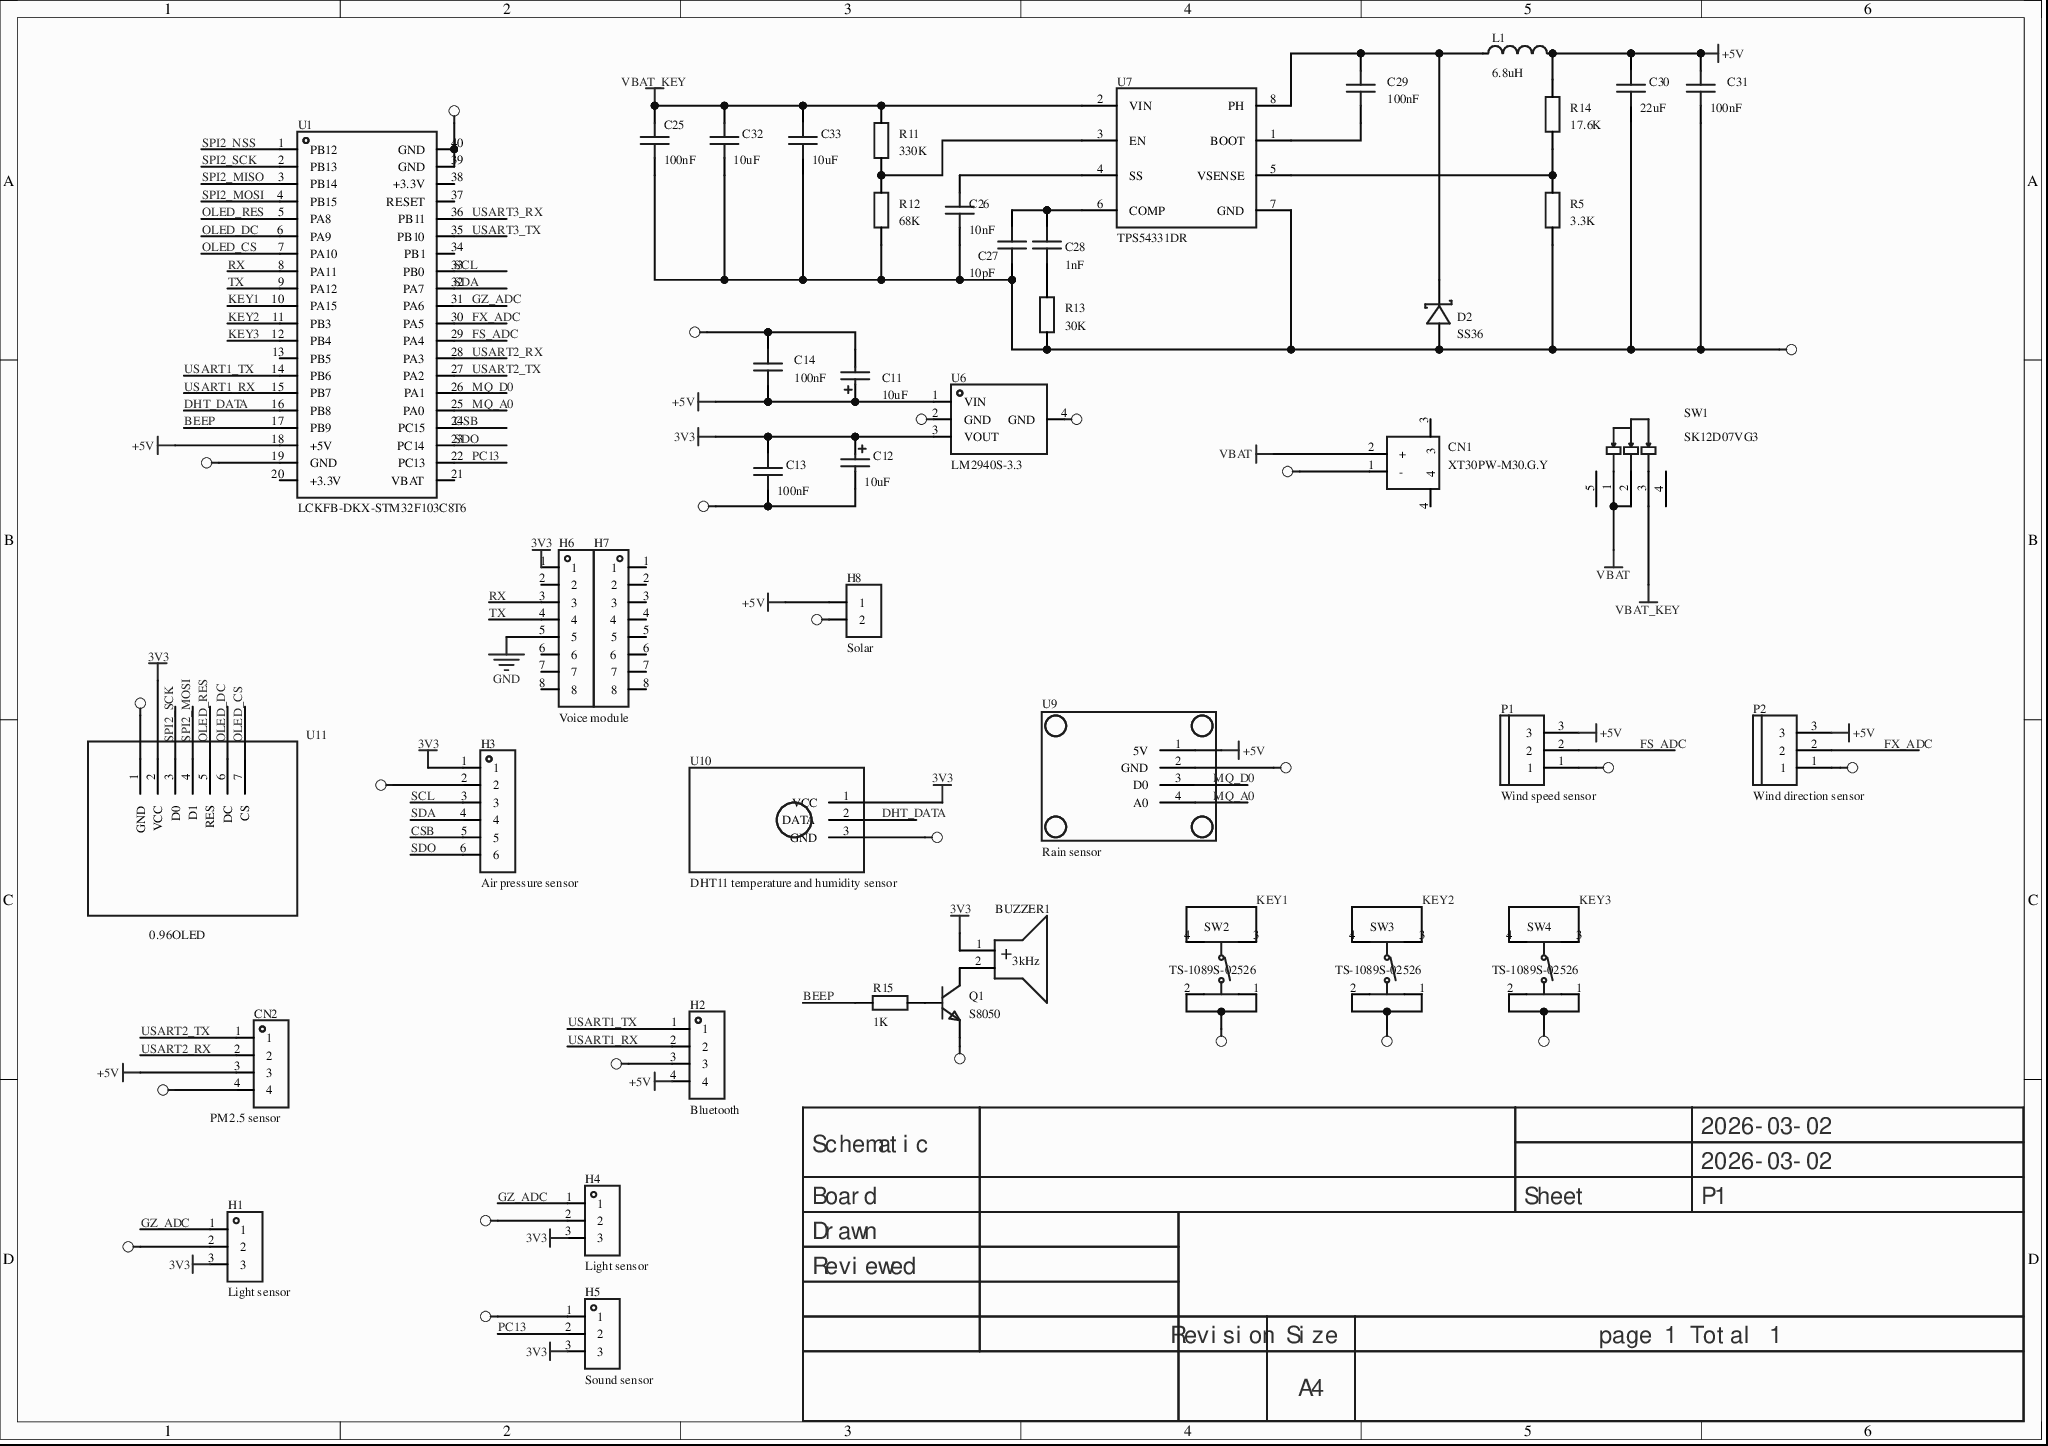
[diagram p0: MISC64781-3.schdoc]
# Altium project MISC64781-2.PrjPcb
1 sheet, 45 parts. Net scope: global (net labels, ports and power ports of the same name join across sheets).
Board file: MISC64781.pcbdoc

## Sheet MISC64781-3.schdoc
size 297 x 209 mm; Version: V1.0; @Project Name: MISC64781; @Page Count: 1; @Update Date: 2026-03-02; @Create Date: 2026-03-02; @Schematic Name: MISC64781; @Page No: 1; @Create Time: 18:43:32; @Update Time: 20:38:21; @Board Name: MISC64781

### Parts
BUZZER1  3kHz  [BUZ-TH_BD9.0-P5.00-D0.6-FD]
C11  10uF  [CASE-A_3216]
C12  10uF  [CASE-A_3216]
C13  100nF  [C0603]
C14  100nF  [C0603]
C25  100nF  [C0603]
C26  10nF  [C0603]
C27  10pF  [C0603]
C28  1nF  [C0603]
C29  100nF  [C0603]
C30  22uF  [C0603]
C31  100nF  [C0603]
C32  10uF  [C0805]
C33  10uF  [C0805]
CN1  XT30PW-M30.G.Y  [CONN-TH_XT30PW-M]
CN2  PM2.5 sensor  [CONN-TH_4P-P1.50_HCTL_HC-ZH1.5-4AW]
D2  SS36  [SMA_L4.3-W2.6-LS5.2-RD]
H1  Light sensor  [HDR-TH_3P-P2.54-V-F]
H2  Bluetooth  [HDR-TH_4P-P2.54-V-F]
H3  Air pressure sensor  [HDR-TH_6P-P2.54-V-F]
H4  Light sensor  [HDR-TH_3P-P2.54-V-F]
H5  Sound sensor  [HDR-TH_3P-P2.54-V-F]
H6  Voice module  [HDR-TH_8P-P2.54-V-F-1]
H7  (no value)  [HDR-TH_8P-P2.54-V-F-1]
H8  Solar  [HDR-TH_2P-P2.54-V-F]
L1  6.8uH  [IND-SMD_L7.0-W6.6]
P1  Wind speed sensor  [CONN-TH_3P-P5.00_WJ500V-5.08-3P]
P2  Wind direction sensor  [CONN-TH_3P-P5.00_WJ500V-5.08-3P]
Q1  S8050  [SOT-23-3_L2.9-W1.3-P1.90-LS2.3-BR]
R5  3.3K  [R0603]
R11  330K  [R0603]
R12  68K  [R0603]
R13  30K  [R0603]
R14  17.6K  [R0603]
R15  1K  [R0603]
SW1  SK12D07VG3  [SW-TH_SK12D07VG3]
SW2  TS-1089S-02526  [SW-SMD_4P-L4.2-W3.3-P2.15-LS5.1]
SW3  TS-1089S-02526  [SW-SMD_4P-L4.2-W3.3-P2.15-LS5.1]
SW4  TS-1089S-02526  [SW-SMD_4P-L4.2-W3.3-P2.15-LS5.1]
U1  LCKFB-DKX-STM32F103C8T6  [CONN-TH_L53.3-W22.9_STM32F103C8T6-CARD]
U6  LM2940S-3.3  [SOT-223-3_L6.5-W3.4-P2.30-LS7.0-BR]
U7  TPS54331DR  [SOIC-8_L5.0-W4.0-P1.27-LS6.0-BL]
U9  Rain sensor  [MQ-2烟雾传感器模块]
U10  DHT11 temperature and humidity sensor  [DHT11温湿度模块]
U11  0.96OLED  [0.96寸OLED]

### Nets
3V3: BUZZER1.1(+) C12.1 C13.2 H1.3 H3.1 H4.3 H5.3 H6.1 U6.3(VOUT) U10.1(VCC) U11.2(VCC)
+5V: C11.1 C14.1 C30.2 C31.2 CN2.3 H2.4 H8.1 L1.2 P1.3 P2.3 R14.2 U1.18(+5V) U6.1(VIN) U9.1(5V)
GND: H6.5
PGND: C11.2 C12.2 C13.1 C14.2 C25.1 C26.1 C27.1 C30.1 C31.1 C32.1 C33.1 CN1.1(-) CN2.4 D2.2(A) H1.2 H2.3 H3.2 H4.2 H5.1 H8.2 P1.1 P2.1 Q1.2(E) R5.1 R12.1 R13.1 SW2.1 SW2.2 SW3.1 SW3.2 SW4.1 SW4.2 U1.19(GND) U1.39(GND) U1.40(GND) U6.2(GND) U6.4(GND) U7.7(GND) U9.2(GND) U10.3(GND) U11.1(GND)
VBAT: CN1.2(+) SW1.1 SW1.2
VBAT_KEY: C25.2 C32.2 C33.2 R11.2 SW1.3 U7.2(VIN)
BEEP: R15.1 U1.17(PB9)
CSB: H3.5 U1.24(PC15)
DHT_DATA: U1.16(PB8) U10.2(DATA)
FS_ADC: P1.2 U1.29(PA4)
FX_ADC: P2.2 U1.30(PA5)
GZ_ADC: H1.1 H4.1 U1.31(PA6)
KEY1: SW2.3 SW2.4 U1.10(PA15)
KEY2: SW3.3 SW3.4 U1.11(PB3)
KEY3: SW4.3 SW4.4 U1.12(PB4)
MQ_A0: U1.25(PA0) U9.4(A0)
MQ_D0: U1.26(PA1) U9.3(D0)
OLED_CS: U1.7(PA10) U11.7(CS)
OLED_DC: U1.6(PA9) U11.6(DC)
OLED_RES: U1.5(PA8) U11.5(RES)
PC13: H5.2 U1.22(PC13)
RX: H6.3 U1.8(PA11)
SCL: H3.3 U1.33(PB0)
SDA: H3.4 U1.32(PA7)
SDO: H3.6 U1.23(PC14)
SPI2_MISO: U1.3(PB14)
SPI2_MOSI: U1.4(PB15) U11.4(D1)
SPI2_NSS: U1.1(PB12)
SPI2_SCK: U1.2(PB13) U11.3(D0)
TX: H6.4 U1.9(PA12)
USART1_RX: H2.2 U1.15(PB7)
USART1_TX: H2.1 U1.14(PB6)
USART2_RX: CN2.2 U1.28(PA3)
USART2_TX: CN2.1 U1.27(PA2)
USART3_RX: U1.36(PB11)
USART3_TX: U1.35(PB10)
NetBUZZER1_2: BUZZER1.2(-) Q1.3(C)
NetC26_2: C26.2 U7.4(SS)
NetC27_2: C27.2 C28.2 U7.6(COMP)
NetC28_1: C28.1 R13.2
NetC29_1: C29.1 U7.1(BOOT)
NetC29_2: C29.2 D2.1(K) L1.1 U7.8(PH)
NetQ1_1: Q1.1(B) R15.2
NetR5_2: R5.2 R14.1 U7.5(VSENSE)
NetR11_1: R11.1 R12.2 U7.3(EN)

Not connected (* = marked no-connect by the designer): CN1 3* 4*; H6 2 6 7 8; H7 1 2 3 4 5 6 7 8; SW1 4* 5*; U1 13(PB5) 20(+3.3V)* 21(VBAT)* 34(PB1) 37(RESET)* 38(+3.3V)*

### Notes on the sheet
- 2026-03-02
- Schematic
- Board
- Sheet
- P1
- Drawn
- Reviewed
- Revision
- Size
- A4
- page 1 Total 1

### Library data of the parts
BUZZER1 = HNB09A03: Drive: active (built-in driver circuit); type: electromagnetic; frequency: 3kHz; SPL: 85dB;; Manufacturer: 华能; AddInBom: yes; ModelId: 13273335caac486e928bafb4d9fdf12d; ModelName: BUZ-TH_D9.0-H5.5-P5.0; ModelTransform: 354.33,354.33,0,90,0,0,-0.005,0,-177.165; Voltage - Supply: 1.5V~4.5V; Current Consumption: 30mA; Symbol: HNB09A03; Device: HNB09A03; LCSC Part Name: 电磁式有源一体蜂鸣器HNB09A03; SupplierPart: C96102; ManufacturerPart: HNB09A03; Supplier Footprint: 插件,D=9mm; JLCPCB Part Class: Extended Part; Datasheet: https://example.com/upload/public/pdf/source/20241128/61C4C8C3938BB25F7C38FBE94CCE8DCF.pdf; Supplier: LCSC; ConvertToPcb: yes; FootprintName: BUZ-TH_BD9.0-P5.00-D0.6-FD; Driver Circuitry: Active (built-in driver circuit); Technology: Electromagnetic; Value: 3kHz; Sound Pressure Level(SPL): 85dB; Diameter(φD): 9mm; Length: -; Width: -; Height: 5.5mm; Operating Temperature: -20℃~+70℃
C11 C12 = TAJA106K010RNJ: Capacitance: 10uF; tolerance: ±10%; rated voltage: 10V; ESR: 3Ω@100kHz;; Manufacturer: Kyocera AVX; Symbol: TAJC106K016RNJ; AddInBom: yes; ModelId: 803ac3def75e4c7cb895540fe23dd6a1; ModelTransform: 125.984,62.992,0,0,0,0,0,0,0; Device: TAJA106K010RNJ; LCSC Part Name: 10uF ±10% 10V; SupplierPart: C7177; ManufacturerPart: TAJA106K010RNJ; Supplier Footprint: CASE-A-3216; JLCPCB Part Class: Extended Part; Datasheet: https://example.com/upload/public/pdf/source/20160107/1457707750344.pdf; Supplier: LCSC; ConvertToPcb: yes; FootprintName: CASE-A_3216; ModelName: CASE-A_3216; Value: 10uF; Tolerance: ±10%; Rated Voltage: 10V; Equivalent Series Resistance(ESR): 3Ω@100kHz; Operating Temperature: -55℃~+125℃
C13 C14 C25-C31 = CAP_0603: ConvertToPcb: yes; SymbolName: CapAcitance; ModelId: ac125912035d415993ca9572d50418b1; ModelName: C0603_L1.6-W0.8-H0.8; ModelTransform: 62.992,31.496,0,0,0,0,0,0,0; Device: CAP_0603; AddInBom: yes; Supplier Footprint: 0603; FootprintName: C0603
  C13 C14 C25 C29 C31: Value: 100nF
  C26: Value: 10nF
  C27: Value: 10pF
  C28: Value: 1nF
  C30: Value: 22uF
C32 C33 = GRM21BR61H106KE43L: Capacitance: 10uF; tolerance: ±10%; rated voltage: 50V; dielectric (temperature coefficient): X5R;; Manufacturer: muRata(村田); AddInBom: yes; ModelId: 1ba041120af144c991958decab20d241; ModelName: C0805_L2.0-W1.3-H1.3; ModelTransform: 78.74,51.181,0,0,0,0,0,0.0005,0; Symbol: CapAcitance; Device: GRM21BR61H106KE43L; LCSC Part Name: 10uF ±10% 50V; SupplierPart: C440198; ManufacturerPart: GRM21BR61H106KE43L; Supplier Footprint: 0805; JLCPCB Part Class: Basic Part; Datasheet: https://example.com/upload/public/pdf/source/20230811/95AAE0C9AF55EDC31B7A4D8B733F534E.pdf; Supplier: LCSC; ConvertToPcb: yes; FootprintName: C0805; Value: 10uF; Tolerance: ±10%; Voltage Rated: 50V; Temperature Coefficient: X5R
CN1 = XT30PW-M30.G.Y: Category: -; type 1: -;; Manufacturer: AMASS(艾迈斯); AddInBom: yes; ModelId: 722652c2597f41cd937322584dc4b29b; ModelTransform: 523.621,549.2115,0,0,0,0,-0.005,-39.568,-78.74; RatedVoltage: DC 500V; InterfaceType: Male; RatedCurrent: 15A; RecommendedWireGauge: 16/18/20AWG; contact resistance: 1.2mΩ; specifications: 2pin; Symbol: XT30PW-M; Device: XT30PW-M30.G.Y; LCSC Part Name: AMASS(艾迈斯)航模插头 卧式弯脚 XT30PW-M公头; SupplierPart: C431092; ManufacturerPart: XT30PW-M30.G.Y; Supplier Footprint: -; JLCPCB Part Class: Extended Part; Datasheet: https://example.com/upload/public/pdf/source/20220222/6A9F22F7850E25B33E1BE430ADF8560B.pdf; Supplier: LCSC; ConvertToPcb: yes; FootprintName: CONN-TH_XT30PW-M; ModelName: CONN-TH_XT30PW-M; Power: -; Output: -; Input: -; Size: -; Interface: -; Type: RC plug; Colour: -; MaximumCurrent: -; Type1: -; NumberOfUSBHoles: -; MetalMaterial: -; InsulationMaterial: -; FlameRetardantGrade: -; Belt length: -
CN2 = HC-ZH1.5-4AW: Pin structure: 1x4P; pitch: 1.5mm; mounting: right angle; reference series: ZH; total PIN count: 4P; rows: 1; PINs per row: 4; row spacing: -; rated current: 1A; contact material: brass; contact plating: tin; operating temperature range: -25℃~+85℃;; Manufacturer Part: PM2.5传感器; Manufacturer: HCTL(华灿天禄); 3D Model: cc452e99891a49a2a6199bd4a3f9b2fa; 3D Model Transform: 295.275,196.85,0,0,0,0,0,-88.583,-98.425; Number of PINs Per Row: 4; Rated Voltage (Max): 100V; Plastic Material: PBT; Flame Retardant Rating: UL94V-0; Supplementary Features: Formed K pins; Z-Height of the Board: 3.7mm; X-Length of Bottom Edge on Board (Spacing Line): 7.5mm; AddInBom: yes; Symbol: HC-ZH1.5-4AW; Device: HC-ZH1.5-4AW; LCSC Part Name: 1x4P 间距:1.5mm 弯插 系列:ZH; Supplier Part: C2845567; Supplier Footprint: 弯插,P=1.5mm; JLCPCB Part Class: Extended library; Datasheet: https://example.com/upload/public/pdf/source/20230711/CEA84C90BC30863458C9BDB0466F53F6.pdf; Supplier: LCSC; Pins Structure: 1x4P; Pitch: 1.5mm; Mounting Style: Right angle; Reference Series: ZH; Number of Pins: 4P; Number of Rows: 1; Row Spacing: -; Current Rating (Max): 1A; Contact Material: Brass; Contact Plating: Tin; Operating Temperature Range: -25℃~+85℃; Colour: -; Y-Width of Bottom Edge on Board: -; ConvertToPcb: yes; FootprintName: CONN-TH_4P-P1.50_HCTL_HC-ZH1.5-4AW; ModelName: CONN-TH_4P-P1.50_HCTL_HC-ZH1.5-4AW
D2 = SS36_C16015: Diode configuration: single; forward voltage (Vf): 700mV@3A; DC reverse voltage (Vr): 60V; rectified current: 3A;; Manufacturer: MDD(辰达半导体); AddInBom: yes; ModelId: 7ed2c9d0a4a74bbdbba07ab4052caf5b; ModelTransform: 185.039,102.362,0,0,0,0,0,0,0; Reverse Leakage Current (Ir): 500uA@60V; Symbol: SS36; Device: SS36_C16015; LCSC Part Name: 电压:60V 电流:3A; SupplierPart: C16015; ManufacturerPart: SS36; Supplier Footprint: SMA(DO-214AC); JLCPCB Part Class: Extended library; Datasheet: https://example.com/upload/public/pdf/source/20240805/AA9E0521C2CA06C1D9DEDE82C98F4769.pdf; Supplier: LCSC; ConvertToPcb: yes; FootprintName: SMA_L4.3-W2.6-LS5.2-RD; ModelName: SMA_L4.3-W2.6-LS5.2-RD; Diode Configuration: Single; Forward Voltage (Vf@If): 700mV@3A; Reverse Voltage (Vr): 60V; Rectified Current: 3A
H1 = PM254V-11-03-H85: Socket structure: 1x3P; pitch: 2.54mm; row spacing: -; mounting type: through-hole; rows: single; total holes: 3P; plastic height: -; contact material: brass; contact plating: -;; Manufacturer Part: 光照传感器; Manufacturer: XFCN(兴飞); AddInBom: yes; ModelId: f3b3cc5aae9641bf9e56fc160cef875b; ModelName: HDR2.54-F-LI-1X3P; ModelTransform: 299.9994,100,0,0,0,0,0,0,-118.11; Symbol: PM254V-11-03-H85; Device: PM254V-11-03-H85; LCSC Part Name: 间距:2.54mm 1x3P 直插; SupplierPart: C541850; Supplier Footprint: 插件,P=2.54mm; JLCPCB Part Class: Extended library; Datasheet: https://example.com/upload/public/pdf/source/20200518/C541849_85853D71FC67C51915A806977A588FDA.pdf; Supplier: LCSC; ConvertToPcb: yes; FootprintName: HDR-TH_3P-P2.54-V-F; Holes Structure: 1x3P; Pitch: 2.54mm; Row Spacing: -; Mounting Type: Through-hole; Number of Rows: Single row; Number of Holes: 3P; Insulation Height: -; Contact Material: Brass; Contact Plating: -
H2 = 2.54-1*4P母: Socket structure: 1x4P; pitch: 2.54mm; row spacing: -; round/square hole: square hole; mounting type: through-hole; rows: single; total holes: 4P; rated current: 3A; rated voltage: -; socket direction: top; plastic height: -; contact material: bronze; contact plating: -; operating temperature range: -40℃~+105℃; soldering temperature (max): -;; Manufacturer Part: 蓝牙; Manufacturer: BOOMELE(博穆精密); Symbol: 2.54-1*4P female; AddInBom: yes; ModelId: d187812051054f85879fcaa51a310d8e; ModelTransform: 419.6842,98.464,0,0,0,0,0,0,-118.11; Device: 2.54-1*4P female; LCSC Part Name: 间距:2.54mm 1x4P 直插; SupplierPart: C2718488; Supplier Footprint: 插件,P=2.54mm; JLCPCB Part Class: Extended library; Datasheet: https://example.com/upload/public/pdf/source/20210301/C2718488_F4427B881E42CAA8DDB0B1C12B3A522C.pdf; Supplier: LCSC; ConvertToPcb: yes; FootprintName: HDR-TH_4P-P2.54-V-F; ModelName: HDR-TH_4P-P2.54-V-F; Holes Structure: 1x4P; Pitch: 2.54mm; Row Spacing: -; Circular Hole / Square Hole: Square hole; Mounting Type: Through-hole; Number of Rows: Single row; Number of Holes: 4P; Current Rating (Max): 3A; Voltage Rating (Max): -; Holes Direction: Top; Insulation Height: -; Contact Material: Bronze; Contact Plating: -; Operating Temperature Range: -40℃~+105℃; Soldering Temperature(Max): -
H3 = HDR-F_2.54_1x6P: Symbol: Header-Female-2.54_1x6; ConvertToPcb: yes; ModelId: 0f5bcf94dcda47d085f24cdca1696fe90819f05c4eef4c71ace90d822a990e87; ModelTransform: 619.684,94.488,0,0,0,0,0,0,-125.984; Device: HDR-F_2.54_1x6P; AddInBom: yes; SupplierPart: C40877; Supplier Footprint: 插件; FootprintName: HDR-TH_6P-P2.54-V-F; ModelName: HDR-TH_6P-P2.54-V-F
H4 = PM254V-11-03-H85: Socket structure: 1x3P; pitch: 2.54mm; row spacing: -; mounting type: through-hole; rows: single; total holes: 3P; plastic height: -; contact material: brass; contact plating: -;; Manufacturer Part: 光照传感器; Manufacturer: XFCN(兴飞); 3D Model: f3b3cc5aae9641bf9e56fc160cef875b; 3D Model Transform: 299.9994,100,0,0,0,0,0,0,-118.11; AddInBom: yes; ModelName: HDR2.54-F-LI-1X3P; Symbol: PM254V-11-03-H85; Device: PM254V-11-03-H85; LCSC Part Name: 间距:2.54mm 1x3P 直插; Supplier Part: C541850; Supplier Footprint: 插件,P=2.54mm; JLCPCB Part Class: Extended library; Datasheet: https://example.com/upload/public/pdf/source/20200518/C541849_85853D71FC67C51915A806977A588FDA.pdf; Supplier: LCSC; Holes Structure: 1x3P; Pitch: 2.54mm; Row Spacing: -; Mounting Type: Through-hole; Number of Rows: Single row; Number of Holes: 3P; Insulation Height: -; Contact Material: Brass; Contact Plating: -; ConvertToPcb: yes; FootprintName: HDR-TH_3P-P2.54-V-F
H5 = PM254V-11-03-H85: Socket structure: 1x3P; pitch: 2.54mm; row spacing: -; mounting type: through-hole; rows: single; total holes: 3P; plastic height: -; contact material: brass; contact plating: -;; Manufacturer Part: 声音传感器; Manufacturer: XFCN(兴飞); 3D Model: f3b3cc5aae9641bf9e56fc160cef875b; 3D Model Transform: 299.9994,100,0,0,0,0,0,0,-118.11; AddInBom: yes; ModelName: HDR2.54-F-LI-1X3P; Symbol: PM254V-11-03-H85; Device: PM254V-11-03-H85; LCSC Part Name: 间距:2.54mm 1x3P 直插; Supplier Part: C541850; Supplier Footprint: 插件,P=2.54mm; JLCPCB Part Class: Extended library; Datasheet: https://example.com/upload/public/pdf/source/20200518/C541849_85853D71FC67C51915A806977A588FDA.pdf; Supplier: LCSC; Holes Structure: 1x3P; Pitch: 2.54mm; Row Spacing: -; Mounting Type: Through-hole; Number of Rows: Single row; Number of Holes: 3P; Insulation Height: -; Contact Material: Brass; Contact Plating: -; ConvertToPcb: yes; FootprintName: HDR-TH_3P-P2.54-V-F
H6 H7 = HDR-F_2.54_1x8P: Symbol: Header-Female-2.54_1x8; AddInBom: yes; ModelId: 0f7e4d9227ef4fa08d5469c22cc70cdb0819f05c4eef4c71ace90d822a990e87; ModelName: HDR-F-2.54_1x8; ModelTransform: 799.99844,100,0,0,0,0,0,0,-118.11; Device: HDR-F_2.54_1x8P; ConvertToPcb: yes; FootprintName: HDR-TH_8P-P2.54-V-F-1; SupplierPart: C27438; Supplier Footprint: 插件
H8 = HDR-F_2.54_1x2P: Symbol: Header-Female-2.54_1x2; ConvertToPcb: yes; ModelId: a9450ef445564560a104363b9aacde4e0819f05c4eef4c71ace90d822a990e87; ModelName: HDR-TH_2P-P2.54-F-LI-1X2P; ModelTransform: 215.7476,98.425,0,0,0,0,0,0,-129.921; Device: HDR-F_2.54_1x2P; AddInBom: yes; SupplierPart: C49661; Supplier Footprint: 插件; FootprintName: HDR-TH_2P-P2.54-V-F
L1 = FXL0630-6R8-M: Inductance: 6.8uH; tolerance: ±20%; rated current: 5A; saturation current (Isat): 6A; type: molded inductor;; Manufacturer: cjiang(长江微电); AddInBom: yes; ModelId: 6860c29aec394a38a0f014af7f722a42; ModelName: IND-SMD_L7.0-W6.6-H3.0; ModelTransform: 275.59,259.842,0,0,0,0,0,0,0; DC Resistance (DCR): 48mΩ; Symbol: FXL0630-6R8-M; Device: FXL0630-6R8-M; LCSC Part Name: 6.8uH ±20% 6A; SupplierPart: C167221; ManufacturerPart: FXL0630-6R8-M; Supplier Footprint: SMD,6.6x7mm; JLCPCB Part Class: Extended library; Datasheet: https://example.com/upload/public/pdf/source/20240426/3189EA8206330E2108542F9E34E540E7.pdf; Supplier: LCSC; ConvertToPcb: yes; FootprintName: IND-SMD_L7.0-W6.6; Value: 6.8uH; Tolerance: ±20%; Rated Current: 5A; Saturation Current (Isat): 6A; Type: Molded inductor
P1 = WJ500V-5.08-3P: Structure: 1x3P; pitch: 5.08mm; color: green; mounting: through-hole; rated current: 18A; rated voltage: 250V; rows: 1; wire gauge - AWG: 14~30; wire gauge - mm²: 2.5; PINs per row: 3; operating temperature range: -40℃~+105℃;; Manufacturer Part: 风速传感器; Manufacturer: KANGNEX(康奈克斯电气); Symbol: WJ500V-5.08-3P-14-00A; AddInBom: yes; ModelId: f80d5090781743d49abcb05979f5618f; ModelTransform: 623.621,393.7,0,0,0,0,11.811,-20.315,-177.165; Wire Gauge - mm2: 2.5; Number of PINs Per Row: 3; Device: WJ500V-5.08-3P; LCSC Part Name: 5.08mm 1x3P 排数:1 每排P数:3 直插; SupplierPart: C72334; Supplier Footprint: 插件,P=5.08mm; JLCPCB Part Class: Extended library; Datasheet: https://example.com/upload/public/pdf/source/20191225/C72334_8A5EF831D67650233B6B1E3F2BC06274.pdf; Supplier: LCSC; ConvertToPcb: yes; FootprintName: CONN-TH_3P-P5.00_WJ500V-5.08-3P; ModelName: CONN-TH_3P-P5.00_WJ500V-5.08-3P; Pitch: 5.08mm; Color: Green; Mounting Style: Through-hole; Current Rating (Max): 18A; Voltage Rating (Max): 250V; Number of Pins: 3P; Number of Rows: 1; Wire Gauge - AWG: 14~30; Operating Temperature Range: -40℃~+105℃
P2 = WJ500V-5.08-3P: Structure: 1x3P; pitch: 5.08mm; color: green; mounting: through-hole; rated current: 18A; rated voltage: 250V; rows: 1; wire gauge - AWG: 14~30; wire gauge - mm²: 2.5; PINs per row: 3; operating temperature range: -40℃~+105℃;; Manufacturer Part: 风向传感器; Manufacturer: KANGNEX(康奈克斯电气); Symbol: WJ500V-5.08-3P-14-00A; AddInBom: yes; ModelId: f80d5090781743d49abcb05979f5618f; ModelTransform: 623.621,393.7,0,0,0,0,11.811,-20.315,-177.165; Wire Gauge - mm2: 2.5; Number of PINs Per Row: 3; Device: WJ500V-5.08-3P; LCSC Part Name: 5.08mm 1x3P 排数:1 每排P数:3 直插; SupplierPart: C72334; Supplier Footprint: 插件,P=5.08mm; JLCPCB Part Class: Extended library; Datasheet: https://example.com/upload/public/pdf/source/20191225/C72334_8A5EF831D67650233B6B1E3F2BC06274.pdf; Supplier: LCSC; ConvertToPcb: yes; FootprintName: CONN-TH_3P-P5.00_WJ500V-5.08-3P; ModelName: CONN-TH_3P-P5.00_WJ500V-5.08-3P; Pitch: 5.08mm; Color: Green; Mounting Style: Through-hole; Current Rating (Max): 18A; Voltage Rating (Max): 250V; Number of Pins: 3P; Number of Rows: 1; Wire Gauge - AWG: 14~30; Operating Temperature Range: -40℃~+105℃
Q1 = S8050_C20069125: Transistor type: NPN; collector current (Ic): 500mA; collector-emitter breakdown voltage (Vceo): 25V; power dissipation (Pd): 300mW; DC current gain (hFE): 120@50mA,1.0V;; Manufacturer: 宏嘉诚; AddInBom: yes; ModelId: 5504beb8757f4de79731898ec55d3e54; ModelTransform: 114.173,90.551,0,90,0,0,0,0,0; Transition frequency(fT): 100MHz; Current - Collector Cutoff: 100nA; Vce Saturation(VCE(sat)): 600mV; Symbol: S8050_C20069125; Device: S8050_C20069125; LCSC Part Name: hFE:200-350，丝印:J3Y S8050; SupplierPart: C20069125; ManufacturerPart: S8050; Supplier Footprint: SOT-23; JLCPCB Part Class: Extended Part; Datasheet: https://example.com/upload/public/pdf/source/20250107/343E8B94B5C24D0D65D7D4B70E0B73F6.pdf; Supplier: LCSC; ConvertToPcb: yes; FootprintName: SOT-23-3_L2.9-W1.3-P1.90-LS2.3-BR; ModelName: SOT-23-3_L2.9-W1.3-P1.90-LS2.3-BR; type: NPN; Current - Collector(Ic): 500mA; Collector - Emitter Voltage VCEO: 25V; Pd - Power Dissipation: 300mW; DC Current Gain: 120@50mA,1.0V; Operating Temperature: -55℃~+150℃
R5 R11-R15 = Res_0603: ConvertToPcb: yes; SymbolName: Resistor; ModelId: fc143cca1e79419f9cd78b61e9279f08; ModelTransform: 31.8897,63.7794,0,90,0,0,0,0,0; Device: Res_0603; AddInBom: yes; Supplier Footprint: 0603; FootprintName: R0603; ModelName: R0603
  R5: Value: 3.3K
  R11: Value: 330K
  R12: Value: 68K
  R13: Value: 30K
  R14: Value: 17.6K
  R15: Value: 1K
SW1 = SK12D07VG3: Circuit: SPDT; mounting: side entry; switch color: -; rated current (DC): 500mA; rated voltage (DC): 50V; rated current (AC): -; rated voltage (AC): -; mechanical life: 5 thousand cycles;; Manufacturer: SHOU HAN(首韩); Symbol: SK12D07VG3_C431547; AddInBom: yes; ModelId: 951c2d8cae1a45b4bcf1723179613222; ModelTransform: 342.519,330.708,0,0,0,0,-0.591,-77.99,-118.11; Pin Style: PC pins; Switch Length: 8.7mm; Switch Width: 4.4mm; Switch Height: 4.7mm; Device: SK12D07VG3; LCSC Part Name: 两档位卧式拨动开关,柄长3MM; SupplierPart: C431547; ManufacturerPart: SK12D07VG3; Supplier Footprint: 插件; JLCPCB Part Class: Extended library; Datasheet: https://example.com/upload/public/pdf/source/20190925/C431547_01B93C6F3FA5C09E15F8CCBF4E6DB91A.pdf; Supplier: LCSC; ConvertToPcb: yes; FootprintName: SW-TH_SK12D07VG3; ModelName: SW-TH_SK12D07VG3; Actuator Style: -; Mounting Style: Side entry; Actuator Color: -; Current Rating (DC): 500mA; Voltage Rating (DC): 50V; Current Rating (AC): -; Voltage Rating (AC): -; Mechanical Life: 5 thousand cycles; Operating Temperature: -10℃~+50℃
SW2-SW4 = TS-1089S-02526: Circuit: SPST; button shape: oval button; mounting: surface mount; switch length: 4.2mm; switch width: 3.25mm; switch height: 2.5mm; contact current: 50mA; rated voltage (DC): 12V; with light: -; mechanical life: -;; Manufacturer: XUNPU(讯普); AddInBom: yes; ModelId: 101da67941e24d4e9615179a94fc6132; ModelName: SW-SMD_4P-L4.2-W3.3-H2.5-P2.15-LS5.1; ModelTransform: 204.724,127.9525,0,0,0,0,0,0,0; Symbol: TS-1089S-02526; Device: TS-1089S-02526; LCSC Part Name: 4.2*3.25*2.5mm 立贴 轻触开关; SupplierPart: C455282; ManufacturerPart: TS-1089S-02526; Supplier Footprint: SMD,3.3x4.2mm; JLCPCB Part Class: Extended library; Datasheet: https://example.com/upload/public/pdf/source/20191118/C455282_2E86A26A9CC4FEF4662951C4D45ED672.pdf; Supplier: LCSC; ConvertToPcb: yes; FootprintName: SW-SMD_4P-L4.2-W3.3-P2.15-LS5.1; Actuator Style: Oval button; Mounting Style: Surface mount; Switch Length: 4.2mm; Switch Width: 3.25mm; Switch Height: 2.5mm; Contact Current: 50mA; Voltage Rating (DC): 12V; With Lamp: -; Mechanical Life: -
U1 = LCKFB-DKX-STM32F103C8T6: Manufacturer: 立创开发板; AddInBom: yes; Symbol: LCKFB-DKX-STM32F103C8T6; Device: LCKFB-DKX-STM32F103C8T6; LCSC Part Name: 立创·地阔星-STM32F103C8T6开发板; SupplierPart: C22396880; ManufacturerPart: LCKFB-DKX-STM32F103C8T6; Supplier Footprint: -; JLCPCB Part Class: Extended Part; Datasheet: https://example.com/upload/public/pdf/source/20240801/7EEF69F7480DF7C6DA98696664D658D4.pdf; Supplier: LCSC; ConvertToPcb: yes; FootprintName: CONN-TH_L53.3-W22.9_STM32F103C8T6-CARD
U6 = LM2940S-3.3: Output type: fixed; max input voltage: 30V; output voltage: 3.3V; output current: 1A; PSRR: -; output polarity: positive;; Manufacturer: HTC; AddInBom: yes; ModelId: 925194bf9823436183a3e0b978a8d076; ModelName: SOT-223-4P_L6.5-W3.5-H1.6-LS7.0-P2.30; ModelTransform: 279.89794,255.905,0,180,0,0,-3.9385,-0.0005,0; Number of Outputs: 1; Symbol: LM2940S-3.3; Device: LM2940S-3.3; LCSC Part Name: LM2940S-3.3; SupplierPart: C596335; ManufacturerPart: LM2940S-3.3; Supplier Footprint: SOT-223-3L; JLCPCB Part Class: Extended library; Datasheet: https://example.com/upload/public/pdf/source/20200113/C481672_D5DB35B2CB9893CB5D56608F126E1817.pdf; Supplier: LCSC; ConvertToPcb: yes; FootprintName: SOT-223-3_L6.5-W3.4-P2.30-LS7.0-BR; Output Type: Fixed; Maximum Input Voltage: 30V; Output Voltage: 3.3V; Output Current: 1A; Power Supply Rejection Ratio (PSRR): -; Feature: Thermal shutdown (TSD); overcurrent protection (OCP); Operating Temperature: -40℃~+85℃@(Tj); Output Polarity: Positive
U7 = TPS54331DR: Function type: buck; output type: adjustable; operating voltage: 3.5V~28V; output voltage: -; output current: 3A;; Manufacturer: TI(德州仪器); AddInBom: yes; ModelId: e81d2f7d937b4a6ab1dca543ff5d56a4; ModelName: SOIC-8_L4.9-W3.9-H1.7-LS6.0-P1.27; ModelTransform: 189.751,236.22,0,0,0,0,-0.0005,0.0005,0; Switching Frequency: 570kHz; Synchronous Rectification: No; Number of Outputs: 1; Topology: Buck topology; Quiescent Current (Iq): 1mA; Switch tube (built-in/external): Built-in; Symbol: TPS54331DR; Device: TPS54331DR; LCSC Part Name: 3A, 28V 输入非同步降压转换器; SupplierPart: C9865; ManufacturerPart: TPS54331DR; Supplier Footprint: SOIC-8; JLCPCB Part Class: Extended library; Supplier: LCSC; ConvertToPcb: yes; FootprintName: SOIC-8_L5.0-W4.0-P1.27-LS6.0-BL; Function: Buck; Output Type: Adjustable; Input Voltage: 3.5V~28V; Output Voltage: -; Output Current: 3A; Operating Temperature: -40℃~+150℃@(TJ)
U9 = MQ-2烟雾传感器模块: Device: MQ-2 smoke sensor module; AddInBom: yes; Symbol: MQ-2 smoke sensor module; ConvertToPcb: yes
U10 = DHT11温湿度模块: Device: DHT11 temperature and humidity module; AddInBom: yes; ConvertToPcb: yes; SymbolName: DHT11 temperature and humidity module; FootprintName: DHT11 temperature and humidity module
U11 = 0.96寸OLED: Device: 0.96-inch OLED; AddInBom: yes; ConvertToPcb: yes; SymbolName: 0.96-inch OLED; FootprintName: 0.96-inch OLED